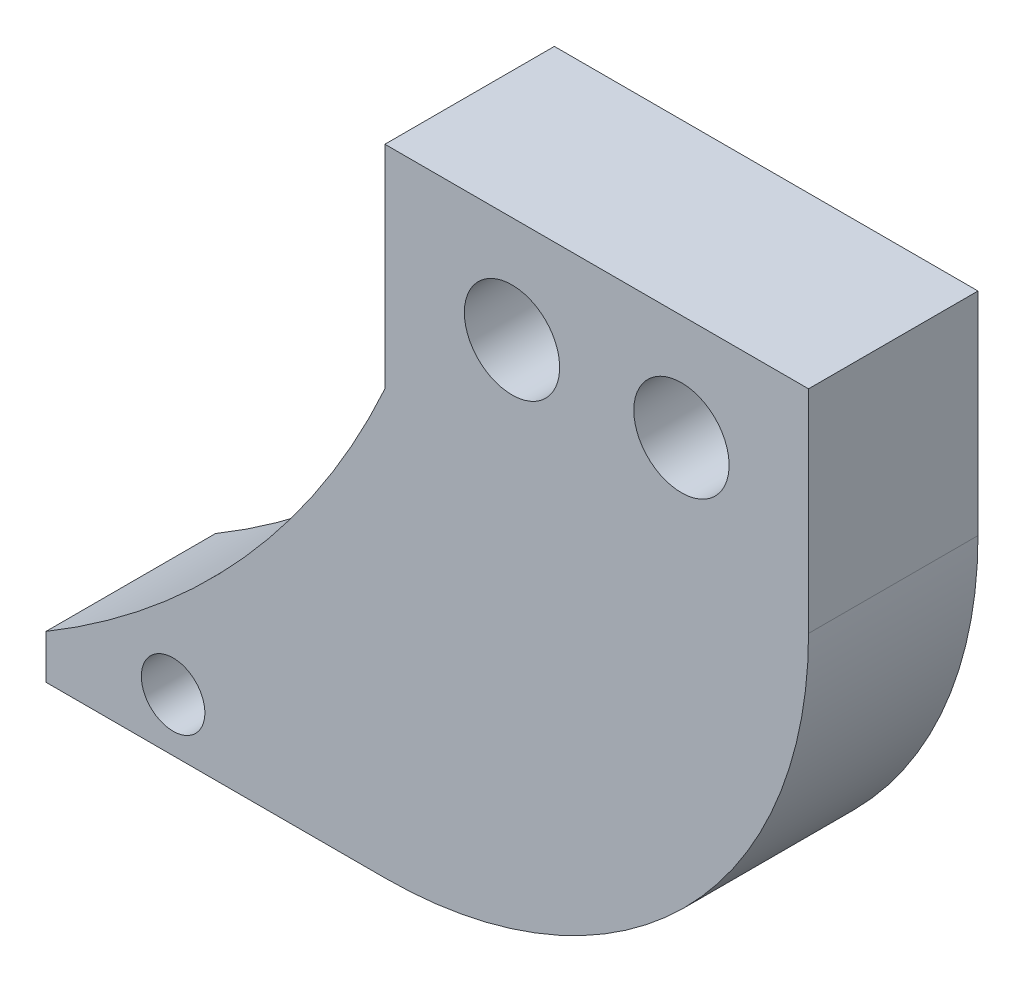
from build123d import *

# Parameters (mm, degrees)
EXTRUDE_1_DEPTH     = 8
SKETCH_2_R          = 1.5
SKETCH_2_R_2        = 2.25
CUT_EXTRUDE_1_DEPTH = 33.213594803


with BuildPart() as part:
    # 草图1 → 凸台-拉伸1 (new body)
    with BuildSketch(Plane.XY):
        with BuildLine():
            Line((-6.680497925, 8.56846473), (13.319502075, 8.56846473))
            Line((13.319502075, 8.56846473), (13.319502075, -1.43153527))
            ThreePointArc((13.319502075, -1.43153527), (7.461637698, -15.573670893), (-6.680497925, -21.43153527))
            Line((-6.680497925, -21.43153527), (-22.680497925, -21.43153527))
            Line((-22.680497925, -21.43153527), (-22.680497925, -19.349484524))
            ThreePointArc((-22.680497925, -19.349484524), (-13.301383699, -11.622002815), (-6.680497925, -1.43153527))
            Line((-6.680497925, -1.43153527), (-6.680497925, 8.56846473))
        make_face()
    extrude(amount=EXTRUDE_1_DEPTH)

    # 草图2 → 切除-拉伸1 (cut, through all)
    with BuildSketch(Plane(origin=(0, 0, 0), x_dir=(-1, 0, 0), z_dir=(0, 0, -1))):
        with Locations((16.680497925, -18.93153527)):
            Circle(SKETCH_2_R)
        with Locations((0.680497925, 3.56846473)):
            Circle(SKETCH_2_R_2)
        with Locations((-7.319502075, 3.56846473)):
            Circle(SKETCH_2_R_2)
    extrude(amount=-CUT_EXTRUDE_1_DEPTH, mode=Mode.SUBTRACT)


solid = part.part
